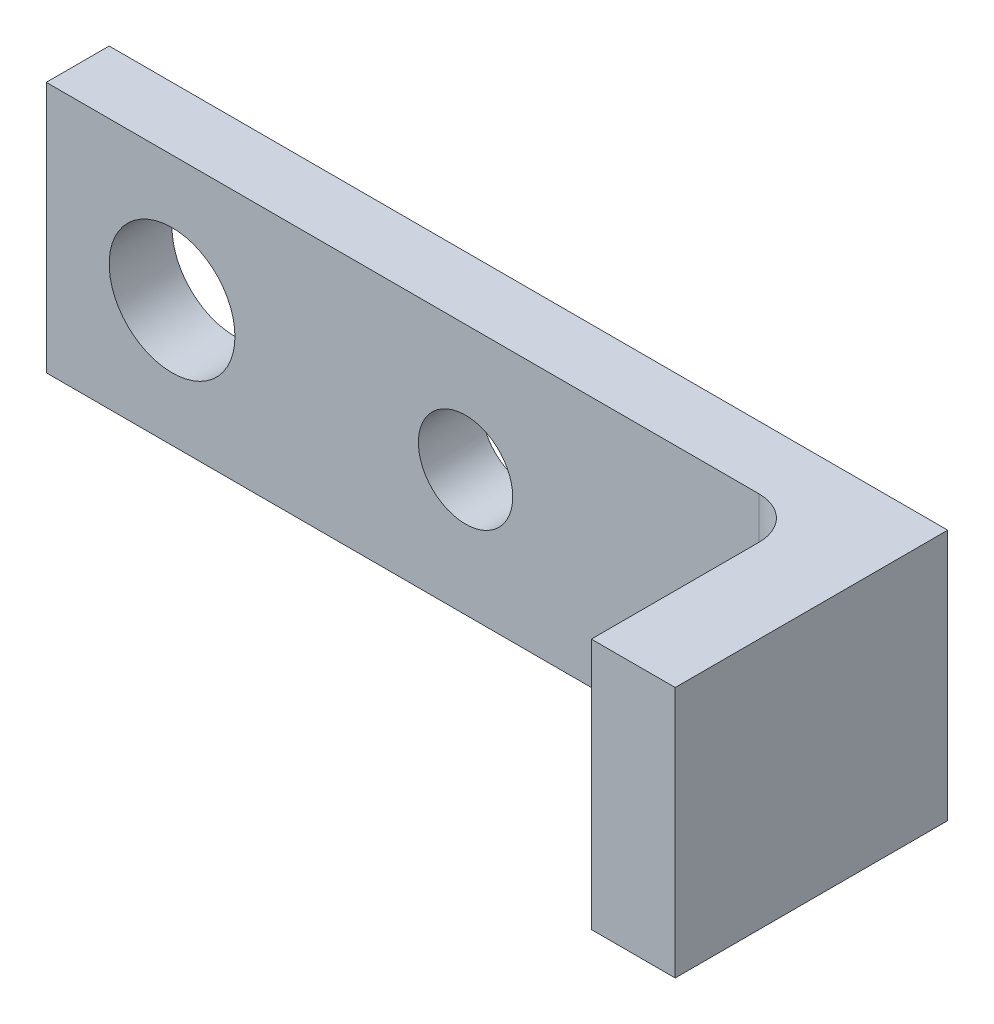
SolidWorks part; units mm, degrees
ref_plane "Front Plane" through (0, 0, 0) normal (0, 0, 1) x (1, 0, 0)
ref_plane "Top Plane" through (0, 0, 0) normal (0, 1, 0) x (1, 0, 0)
ref_plane "Right Plane" through (0, 0, 0) normal (1, 0, 0) x (0, 0, -1)
sketch "Sketch1" plane through (0, 0, 0) normal (0, 0, 1) x (1, 0, 0)
  line L0 (0, 6) -> (40, 6) construction
  line L1 (0, 0) -> (40, 0)
  line L2 (0, 0) -> (0, 12)
  line L3 (0, 12) -> (40, 12)
  line L4 (40, 0) -> (40, 12)
  circle A0 centre (20, 6) radius 2.25
  circle A1 centre (6, 6) radius 3
  dimension "D3" = 4.5
  dimension "D4" = 20
  dimension "D5" = 6
  dimension "D6" = 6
  dimension "D1" = 40
  dimension "D2" = 12
extrude "Boss-Extrude1" add sketch "Sketch1" along normal blind 3
sketch "Sketch2" plane through (0, 0, 3) normal (0, 0, 1) x (1, 0, 0)
  line L0 (40, 12) -> (0, 12) construction
  line L1 (40, 0) -> (36, 0)
  line L2 (40, 0) -> (40, 12)
  line L3 (40, 12) -> (36, 12)
  line L4 (36, 0) -> (36, 12)
  dimension "D1" = 4
extrude "Boss-Extrude2" add sketch "Sketch2" along normal blind 10
fillet "Fillet1" radius 2 1 edges at (36, 6, 3)
